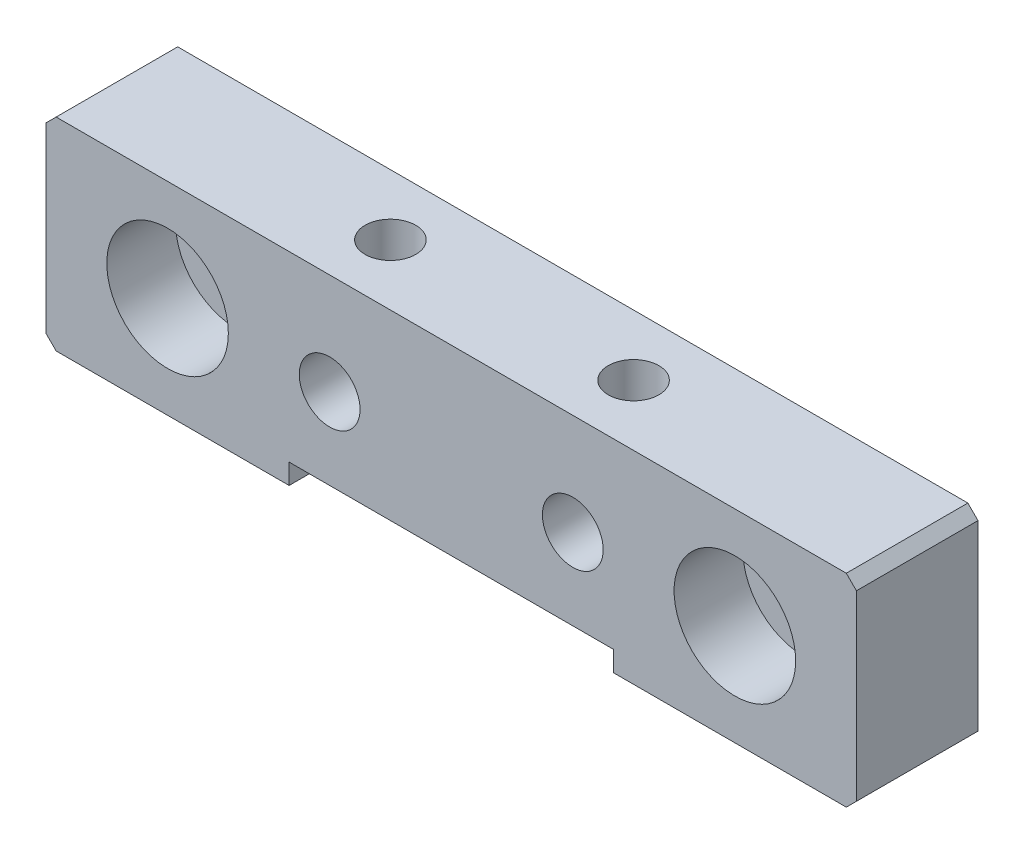
SolidWorks part; units mm, degrees
ref_plane "Front Plane" through (0, 0, 0) normal (0, 0, 1) x (1, 0, 0)
ref_plane "Top Plane" through (0, 0, 0) normal (0, 1, 0) x (1, 0, 0)
ref_plane "Right Plane" through (0, 0, 0) normal (1, 0, 0) x (0, 0, -1)
sketch "Sketch1" plane through (0, 0, 0) normal (0, 0, 1) x (1, 0, 0)
  line L1 (20, -5) -> (-20, -5)
  line L2 (20, -5) -> (20, 5)
  line L3 (20, 5) -> (-20, 5)
  line L4 (-20, -5) -> (-20, 5)
  line L5 (20, -5) -> (-20, 5) construction
  line L6 (20, 5) -> (-20, -5) construction
  point P0 (0, 0)
  dimension "D1" = 10
  dimension "D2" = 40
extrude "Boss-Extrude1" add sketch "Sketch1" along normal blind 6
chamfer "Chamfer1" distance 0.5 angle 45 4 edges at (20, -5, 3) (20, 5, 3) (-20, 5, 3) (-20, -5, 3)
hole_wizard "Hole Size per Socket Head Cap Screw Type1" positions "Sketch3" profile "Sketch2" counterbore size "M3" standard "Gb" end condition through all
sketch "Sketch3" plane through (0, 0, 6) normal (0, 0, 1) x (1, 0, 0)
  line L0 (0, 5) -> (0, -5) construction
  line L1 (19.5, 5) -> (-19.5, 5) construction
  line L2 (-19.5, -5) -> (19.5, -5) construction
  point P0 (-14, 0)
  point P1 (14, 0)
  dimension "D1" = 28
sketch "Sketch2" plane through (-14, 0, 6) normal (1, 0, 0) x (0, -1, 0)
  line L0 (0, 0) -> (0, 6)
  line L1 (0, 6) -> (1.7, 6)
  line L3 (1.7, 6) -> (1.7, 3.4)
  line L4 (1.7, 3.4) -> (3, 3.4)
  line L5 (3, 3.4) -> (3, 0)
  line L7 (3, 0) -> (0, 0)
  line L11 (0, -6.35) -> (0, 107.95) construction
  dimension "通孔孔直径" = 3.4
  dimension "通孔孔深度" = 6
  dimension "柱形沉头孔直径" = 6
  dimension "柱形沉头孔深度" = 3.4
sketch "Sketch4" plane through (0, -5, 0) normal (0, 1, 0) x (1, 0, 0)
  line L0 (19.5, 0) -> (-19.5, 0) construction
  line L1 (8, -6) -> (-8, -6)
  line L2 (8, -6) -> (8, 0)
  line L3 (8, 0) -> (-8, 0)
  line L4 (-8, -6) -> (-8, 0)
  line L5 (8, -6) -> (-8, 0) construction
  line L6 (8, 0) -> (-8, -6) construction
  line L7 (-20, -3) -> (20, -3) construction
  line L8 (-20, -6) -> (-20, 0) construction
  line L9 (20, 0) -> (20, -6) construction
  point P0 (0, -3)
  dimension "D1" = 16
extrude "Cut-Extrude1" cut sketch "Sketch4" along normal blind 1
sketch "Sketch5" plane through (0, 0, 0) normal (0, 0, 1) x (1, 0, 0)
  line L0 (0, 5) -> (0, -4) construction
  line L1 (19.5, 5) -> (-19.5, 5) construction
  line L2 (-8, -4) -> (8, -4) construction
  circle A0 centre (-6, 0) radius 1.5
  circle A1 centre (6, 0) radius 1.5
  dimension "D2" = 3
  dimension "D3" = 3
  dimension "D1" = 12
extrude "Cut-Extrude2" cut sketch "Sketch5" along normal through all
hole_wizard "M3 Tapped Hole1" positions "Sketch7" profile "Sketch6" tap size "M3" standard "GB"
sketch "Sketch7" plane through (0, 5, 0) normal (0, 1, 0) x (-1, 0, 0)
  line L0 (0, 0) -> (0, 10.0496) construction
  line L1 (-19.5, 0) -> (19.5, 0) construction
  point P1 (6, 3)
  point P3 (-6, 3)
  dimension "D1" = 12
  dimension "D2" = 3
sketch "Sketch6" plane through (-6, 5, 3) normal (1, 0, 0) x (0, 0, 1)
  line L0 (0, 0) -> (0, 5.7511)
  line L1 (0, 5.7511) -> (1.25, 5)
  line L2 (1.25, 5) -> (1.25, 0)
  line L5 (1.25, 0) -> (0, 0)
  line L10 (0, 5.7511) -> (-1.25, 5) construction
  line L11 (0, -6.35) -> (0, 107.95) construction
  dimension "螺纹孔钻头直径" = 2.5
  dimension "螺纹孔钻头深度" = 5
  dimension "导头角度" = 118
cosmetic thread "Cosmetic Thread1" parameters "D1"=4.1708, "D2"=3
cosmetic thread "Cosmetic Thread2" parameters "D1"=4.1708, "D2"=3
